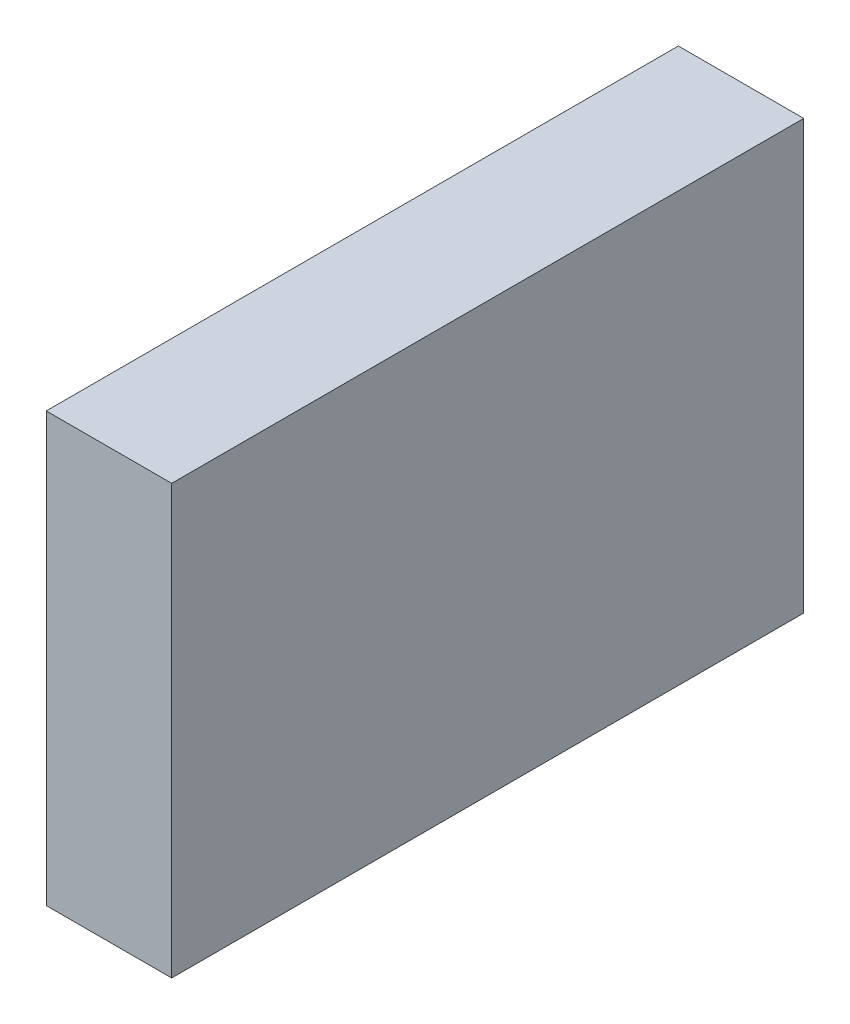
from build123d import *

# Parameters (mm, degrees)
SKETCH2_W           = 25
SKETCH2_H           = 126
BOSS_EXTRUDE1_DEPTH = 42.7


with BuildPart() as part:
    # Sketch2 → Boss-Extrude1 (new, symmetric)
    with BuildSketch(Plane(origin=(0, 0, 0), x_dir=(1, 0, 0), z_dir=(0, 1, 0))):
        Rectangle(SKETCH2_W, SKETCH2_H)
    extrude(amount=BOSS_EXTRUDE1_DEPTH, both=True)


solid = part.part
